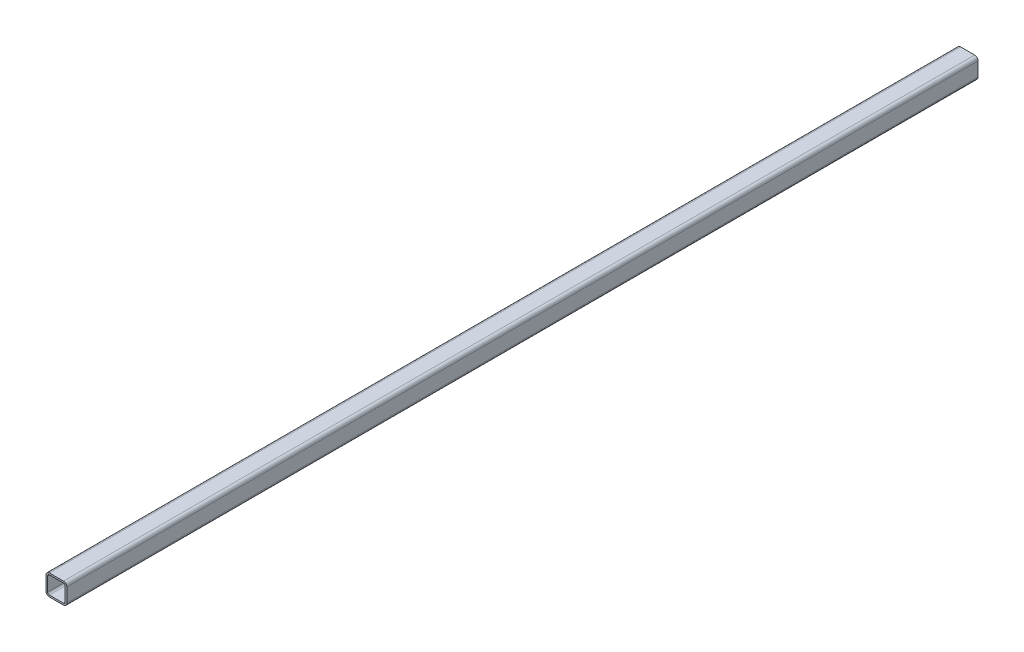
SolidWorks part; units mm, degrees
material "Q235"
ref_plane "Plane1" through (0, 0, 0) normal (0, 0, 1) x (1, 0, 0)
ref_plane "Plane2" through (0, 0, 0) normal (0, 1, 0) x (1, 0, 0)
ref_plane "Plane3" through (0, 0, 0) normal (1, 0, 0) x (0, 0, -1)
sketch "Sketch1" plane through (0, 0, 0) normal (0, 0, 1) x (1, 0, 0)
  line L0 (-8.5, -10.5) -> (8.5, -10.5)
  line L1 (-10.5, -8.5) -> (-10.5, 8.5)
  line L2 (8.5, 10.5) -> (-8.5, 10.5)
  line L3 (10.5, 8.5) -> (10.5, -8.5)
  line L4 (-8.5, -12.5) -> (8.5, -12.5)
  line L5 (-12.5, -8.5) -> (-12.5, 8.5)
  line L6 (8.5, 12.5) -> (-8.5, 12.5)
  line L7 (12.5, 8.5) -> (12.5, -8.5)
  arc A0 (12.5, 8.5) -> (8.5, 12.5) centre (8.5, 8.5) ccw
  arc A1 (8.5, -12.5) -> (12.5, -8.5) centre (8.5, -8.5) ccw
  arc A2 (-12.5, -8.5) -> (-8.5, -12.5) centre (-8.5, -8.5) ccw
  arc A3 (-8.5, 12.5) -> (-12.5, 8.5) centre (-8.5, 8.5) ccw
  arc A4 (-8.5, 10.5) -> (-10.5, 8.5) centre (-8.5, 8.5) ccw
  arc A5 (10.5, 8.5) -> (8.5, 10.5) centre (8.5, 8.5) ccw
  arc A6 (8.5, -10.5) -> (10.5, -8.5) centre (8.5, -8.5) ccw
  arc A7 (-10.5, -8.5) -> (-8.5, -10.5) centre (-8.5, -8.5) ccw
  point P0 (0, 12.5)
  point P1 (12.5, 0)
  point P2 (0, -12.5)
  point P3 (-12.5, 0)
  point P4 (-12.5, 12.5)
  point P5 (12.5, 12.5)
  point P6 (12.5, -12.5)
  point P7 (-12.5, -12.5)
  point P8 (0, 0)
extrude "Boss-Extrude1" add sketch "Sketch1" along normal blind 1094
